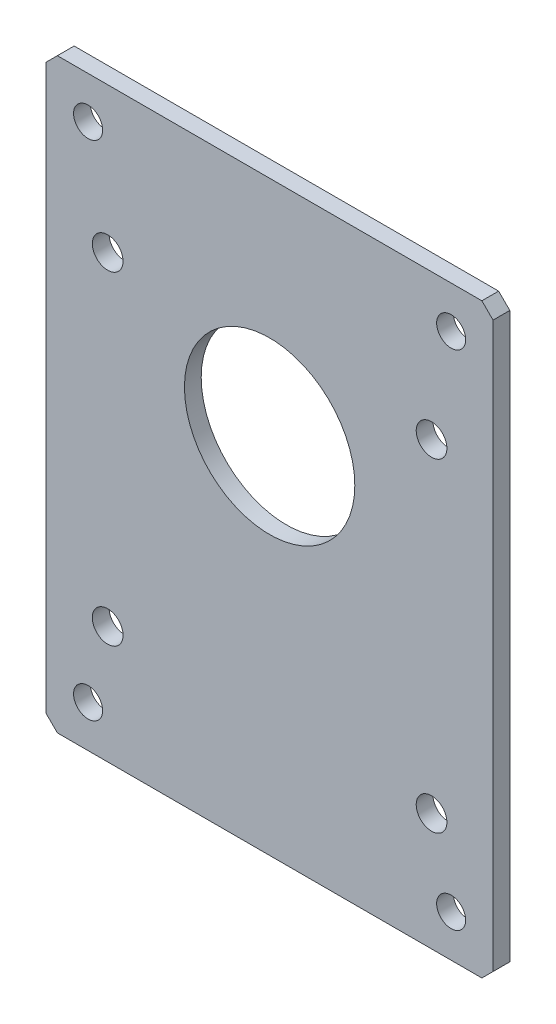
from build123d import *

# Parameters (mm, degrees)
SKETCH1_W             = 80
SKETCH1_H             = 105
BOSS_EXTRUDE1_DEPTH   = 3
SKETCH2_R             = 2.6
SKETCH2_R_2           = 15.25
CUT_EXTRUDE1_DEPTH    = 10
M5_TAPPED_HOLE1_D     = 4.2
M5_TAPPED_HOLE1_DEPTH = 12.4
M5_TAPPED_HOLE1_TIP   = 1.2618073
CHAMFER1_SIZE         = 2
SKETCH6_R             = 2.75
CUT_EXTRUDE3_DEPTH    = 133.037873355


with BuildPart() as part:
    # Sketch1 → Boss-Extrude1 (new body)
    with BuildSketch(Plane.XY):
        with Locations((40, 52.5)):
            Rectangle(SKETCH1_W, SKETCH1_H)
    extrude(amount=BOSS_EXTRUDE1_DEPTH)

    # Sketch2 → Cut-Extrude1 (cut)
    with BuildSketch(Plane.XY.offset(3)):
        with Locations((7.5, 97.5)):
            Circle(SKETCH2_R)
        with Locations((72.5, 97.5)):
            Circle(SKETCH2_R)
        with Locations((7.5, 7.5)):
            Circle(SKETCH2_R)
        with Locations((72.5, 7.5)):
            Circle(SKETCH2_R)
        with Locations((40, 65)):
            Circle(SKETCH2_R_2)
    extrude(amount=-CUT_EXTRUDE1_DEPTH, mode=Mode.SUBTRACT)

    # M5 Tapped Hole1
    with Locations(Plane.XY.offset(3)):
        with Locations((11.008621971, 78.991378029), (68.991378029, 78.991378029), (11.008621971, 21.008621971), (68.991378029, 21.008621971)):
            Hole(M5_TAPPED_HOLE1_D / 2, depth=M5_TAPPED_HOLE1_DEPTH)
            with Locations((0, 0, -(M5_TAPPED_HOLE1_DEPTH + M5_TAPPED_HOLE1_TIP / 2))):  # 118° drill point
                Cone(0, M5_TAPPED_HOLE1_D / 2, M5_TAPPED_HOLE1_TIP, mode=Mode.SUBTRACT)

    # Chamfer1
    chamfer1_edges = [part.edges().sort_by_distance(p)[0] for p in [
        (0, 105, 1.5),
        (80, 105, 1.5),
        (80, 0, 1.5),
        (0, 0, 1.5),
    ]]
    chamfer(chamfer1_edges, length=CHAMFER1_SIZE)

    # Sketch6 → Cut-Extrude3 (cut, through all)
    with BuildSketch(Plane(origin=(0, 0, 0), x_dir=(-1, 0, 0), z_dir=(0, 0, -1))):
        with Locations((-68.991378029, 78.991378029)):
            Circle(SKETCH6_R)
        with Locations((-11.008621971, 78.991378029)):
            Circle(SKETCH6_R)
        with Locations((-68.991378029, 21.008621971)):
            Circle(SKETCH6_R)
        with Locations((-11.008621971, 21.008621971)):
            Circle(SKETCH6_R)
    extrude(amount=-CUT_EXTRUDE3_DEPTH, mode=Mode.SUBTRACT)


solid = part.part
